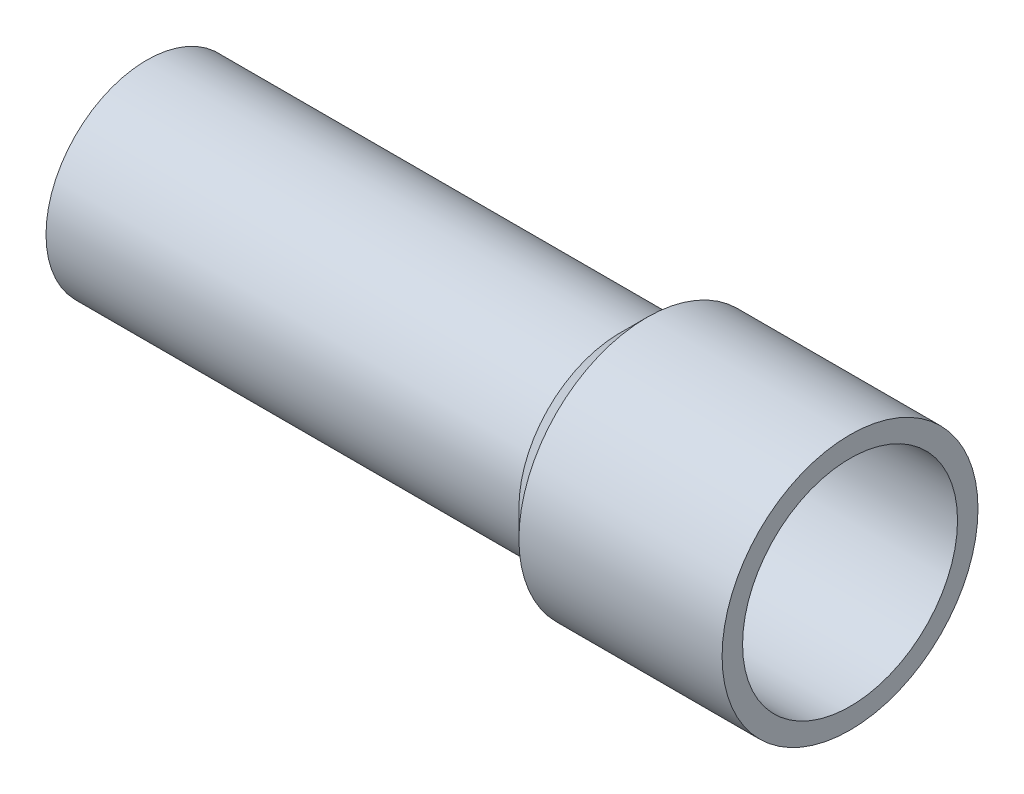
from build123d import *


with BuildPart() as part:
    # Sketch1 → Revolve1 (revolve)
    with BuildSketch(Plane.XY, mode=Mode.PRIVATE) as revolve1_sk:
        Polygon((0, 1.97), (9.24, 1.97), (9.77, 2.5), (13.74, 2.5), (13.74, 2.1), (9.935685425, 2.1), (9.405685425, 1.57), (0, 1.57), align=None)
    revolve(revolve1_sk.sketch.rotate(Axis((0, 0, 0), (1, 0, 0)), 90), axis=Axis((0, 0, 0), (1, 0, 0)))


solid = part.part
